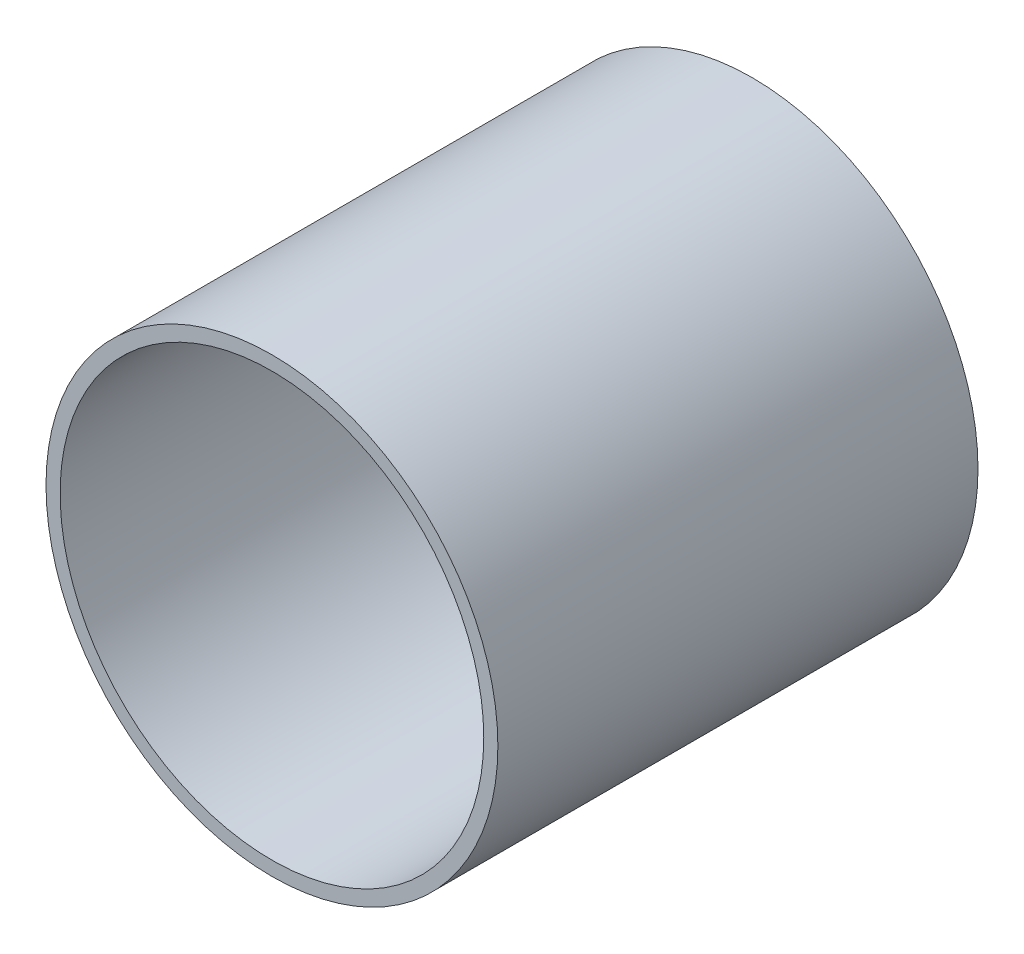
SolidWorks part; units mm, degrees
ref_plane "前视基准面" through (0, 0, 0) normal (0, 0, 1) x (1, 0, 0)
ref_plane "上视基准面" through (0, 0, 0) normal (0, 1, 0) x (1, 0, 0)
ref_plane "右视基准面" through (0, 0, 0) normal (1, 0, 0) x (0, 0, -1)
other "Configuration Table"
sketch "草图1" plane through (0, 0, 0) normal (0, 0, 1) x (1, 0, 0)
  circle A0 centre (0, 0) radius 80
  circle A1 centre (0, 0) radius 75
  dimension "D1" = 160
  dimension "D2" = 150
extrude "凸台-拉伸1" add sketch "草图1" along normal blind 170
